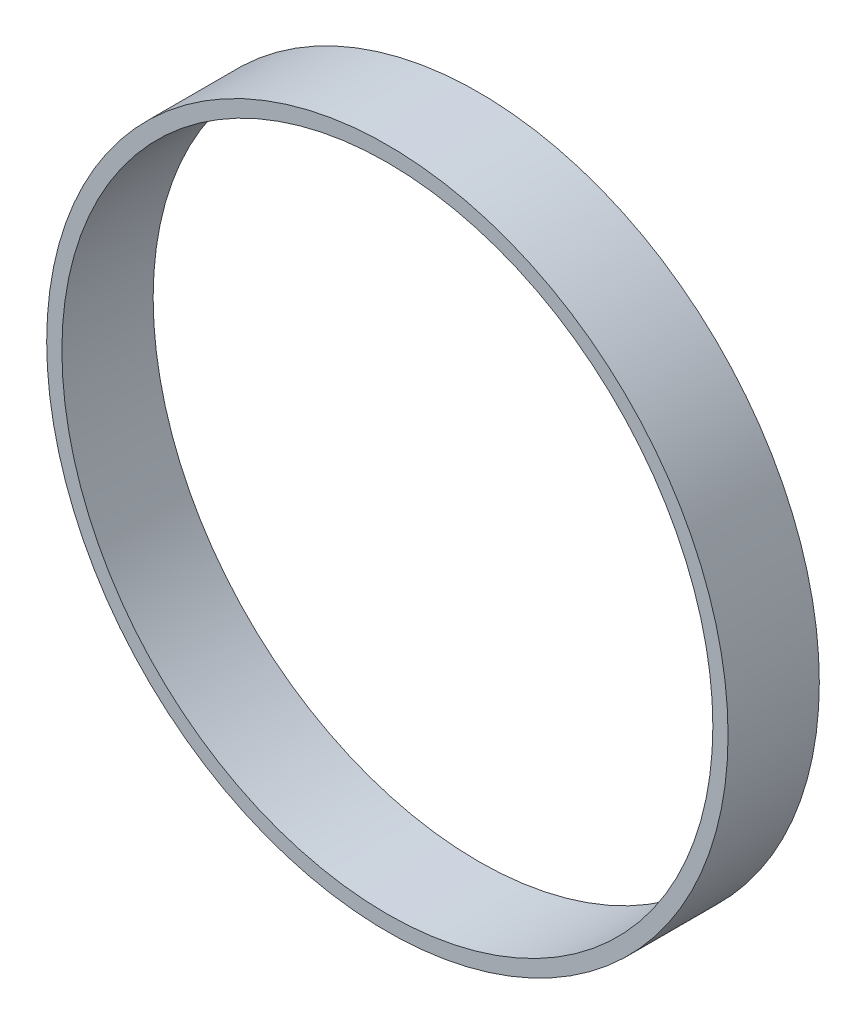
SolidWorks part; units mm, degrees
ref_plane "Front Plane" through (0, 0, 0) normal (0, 0, 1) x (1, 0, 0)
ref_plane "Top Plane" through (0, 0, 0) normal (0, 1, 0) x (1, 0, 0)
ref_plane "Right Plane" through (0, 0, 0) normal (1, 0, 0) x (0, 0, -1)
sketch "Sketch1" plane through (0, 0, 0) normal (0, 0, 1) x (1, 0, 0)
  circle A0 centre (0, 0) radius 56
  circle A1 centre (0, 0) radius 53.5
  dimension "D1" = 112
  dimension "D2" = 2.5
extrude "Boss-Extrude1" add sketch "Sketch1" along normal blind 15
